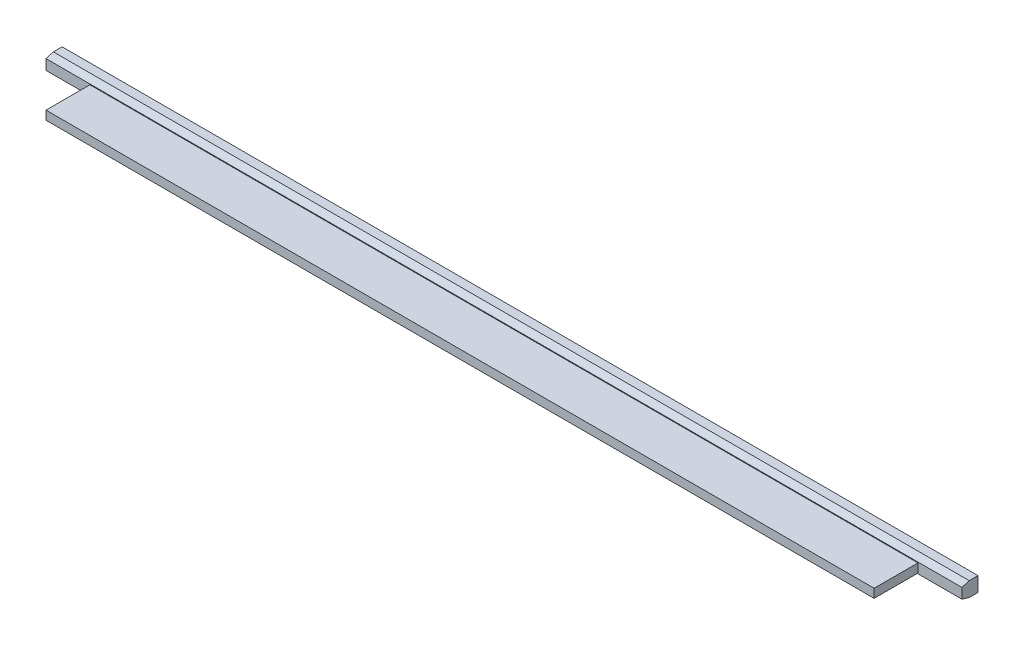
from build123d import *

# Parameters (mm, degrees)
SKETCH1_W           = 313
SKETCH1_H           = 5
BOSS_EXTRUDE1_DEPTH = 5.5
CUT_EXTRUDE1_DEPTH  = 314.058301279
SKETCH2_W           = 283
SKETCH2_H           = 3
BOSS_EXTRUDE2_DEPTH = 15


with BuildPart() as part:
    # Sketch1 → Boss-Extrude1 (new body)
    with BuildSketch(Plane.XY):
        Rectangle(SKETCH1_W, SKETCH1_H)
    extrude(amount=BOSS_EXTRUDE1_DEPTH)

    # Sketch3 → Cut-Extrude1 (cut, through all)
    with BuildSketch(Plane(origin=(156.5, 0, 0), x_dir=(0, 0, -1), z_dir=(1, 0, 0))):
        Polygon((-3, 2.5), (-5.5, 1.75), (-5.5, 2.5), align=None)
        Polygon((-3, -2.5), (-5.5, -1.75), (-5.5, -2.5), align=None)
    extrude(amount=-CUT_EXTRUDE1_DEPTH, mode=Mode.SUBTRACT)

    # Sketch2 → Boss-Extrude2 (add)
    with BuildSketch(Plane.XY.offset(5.5)):
        Rectangle(SKETCH2_W, SKETCH2_H)
    extrude(amount=BOSS_EXTRUDE2_DEPTH)


solid = part.part
